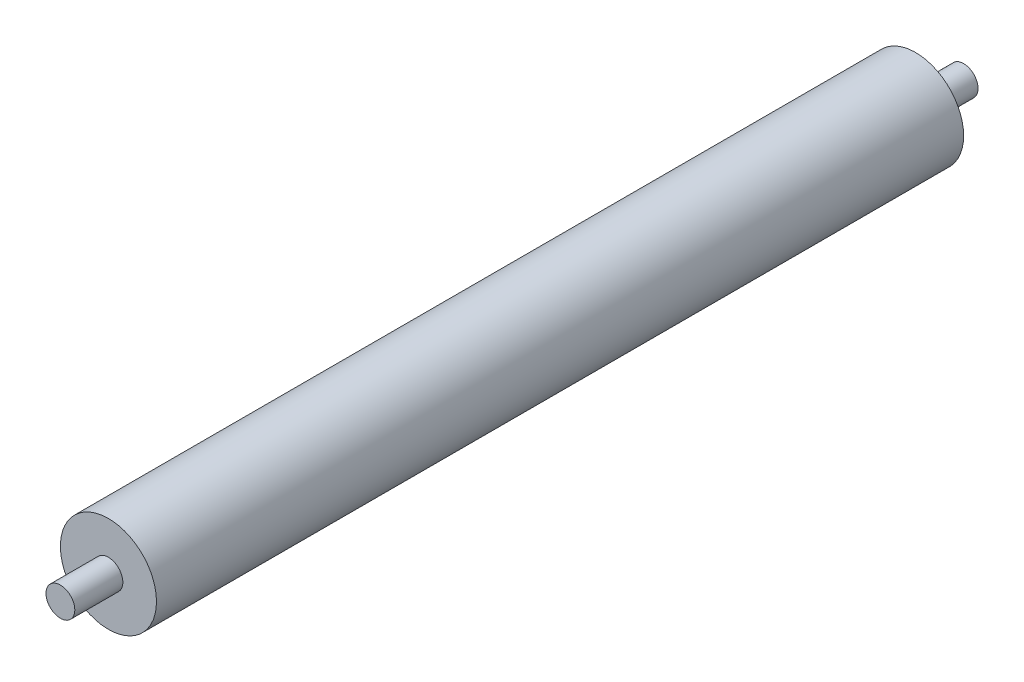
from build123d import *

# Parameters (mm, degrees)
SKETCH_1_R      = 25
EXTRUDE_1_DEPTH = 420
SKETCH_2_R      = 7.5
EXTRUDE_2_DEPTH = 25
EXTRUDE_START   = 25
SKETCH_3_R      = 7.5
EXTRUDE_3_DEPTH = 25


with BuildPart() as part:
    # 草图1 → 凸台-拉伸1 (new body)
    with BuildSketch(Plane.XY):
        Circle(SKETCH_1_R)
    extrude(amount=EXTRUDE_1_DEPTH)

    # 草图2 → 凸台-拉伸2 (add)
    with BuildSketch(Plane.XY.offset(420)):
        Circle(SKETCH_2_R)
    extrude(amount=EXTRUDE_2_DEPTH)

    # 草图3 → 凸台-拉伸3 (add)
    with BuildSketch(Plane(origin=(0, 0, 0), x_dir=(-1, 0, 0), z_dir=(0, 0, -1)).offset(EXTRUDE_START)):
        with Locations(Location((0, 0, 0), (0, 0, 180))):
            Circle(SKETCH_3_R)
    extrude(amount=-EXTRUDE_3_DEPTH)


solid = part.part
